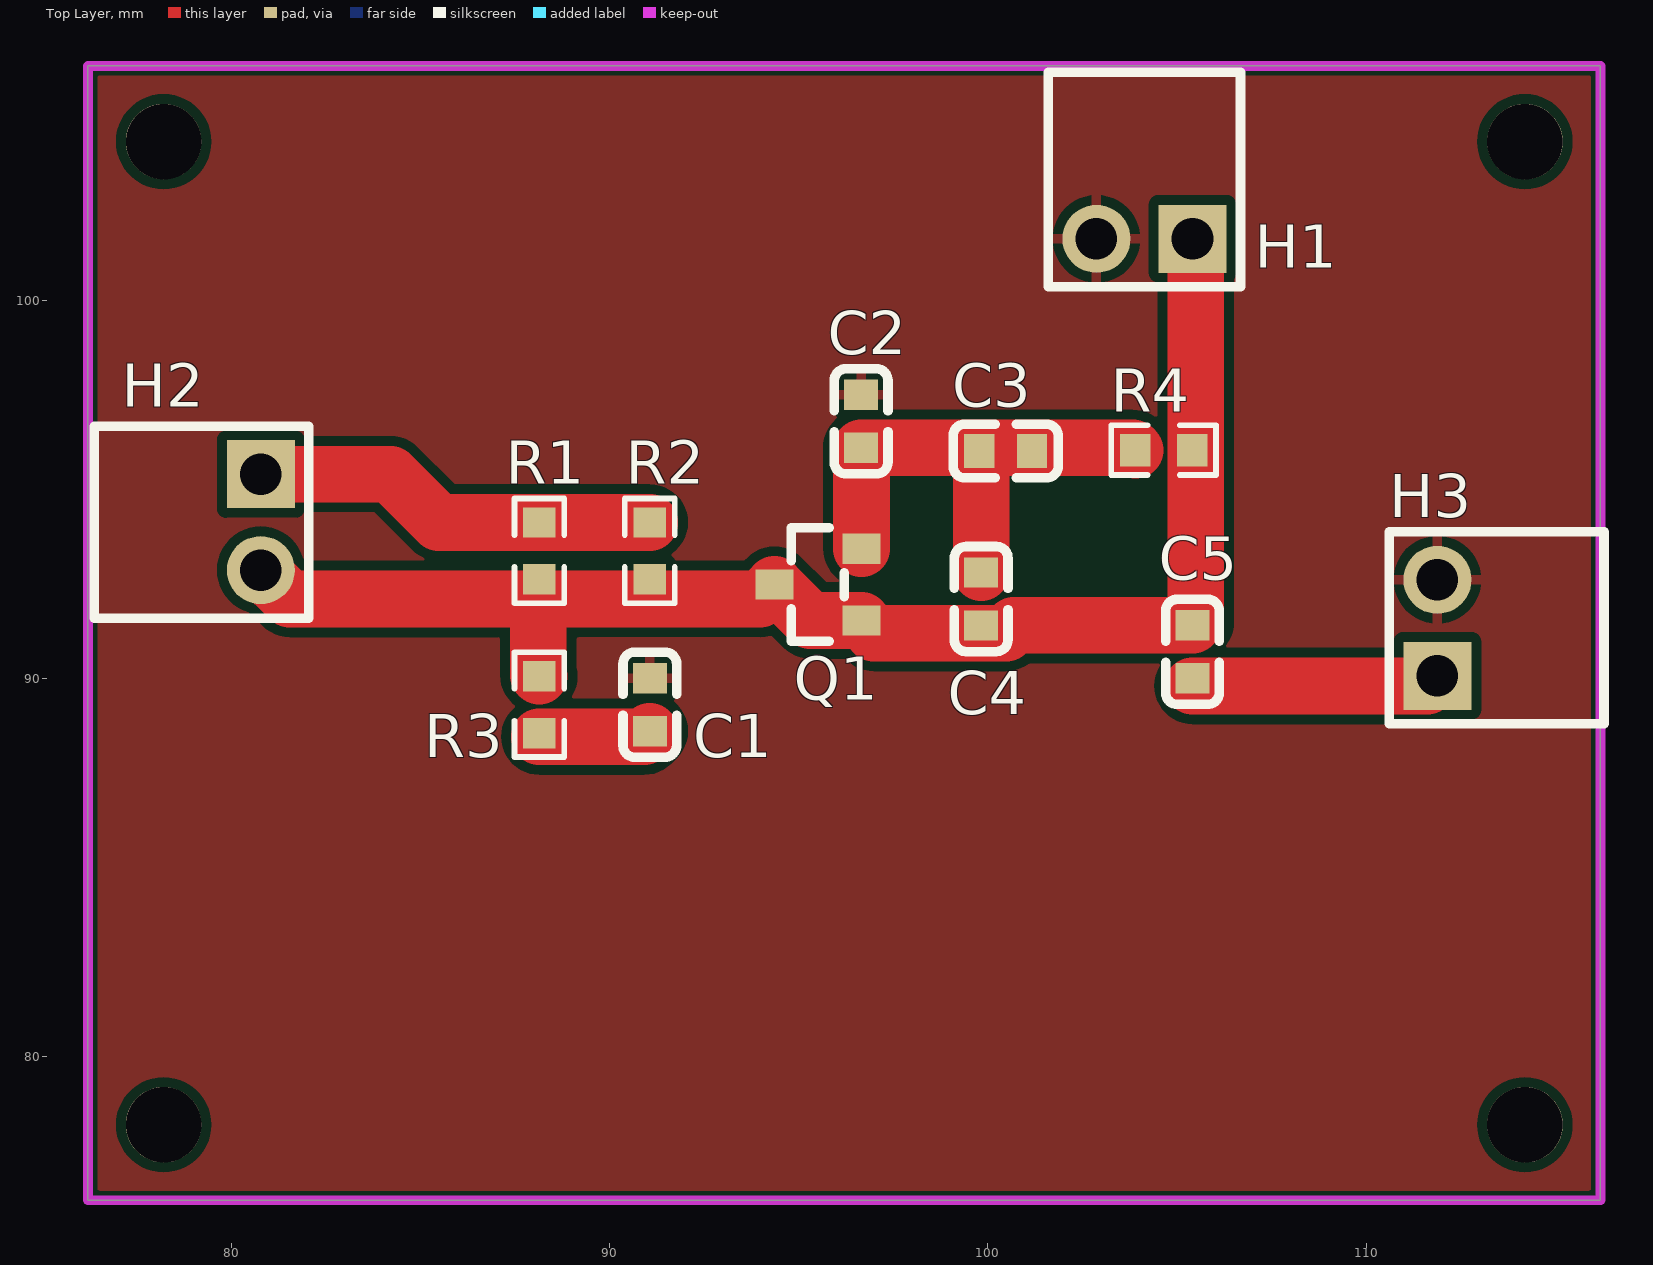
[diagram p0: Top Layer view]
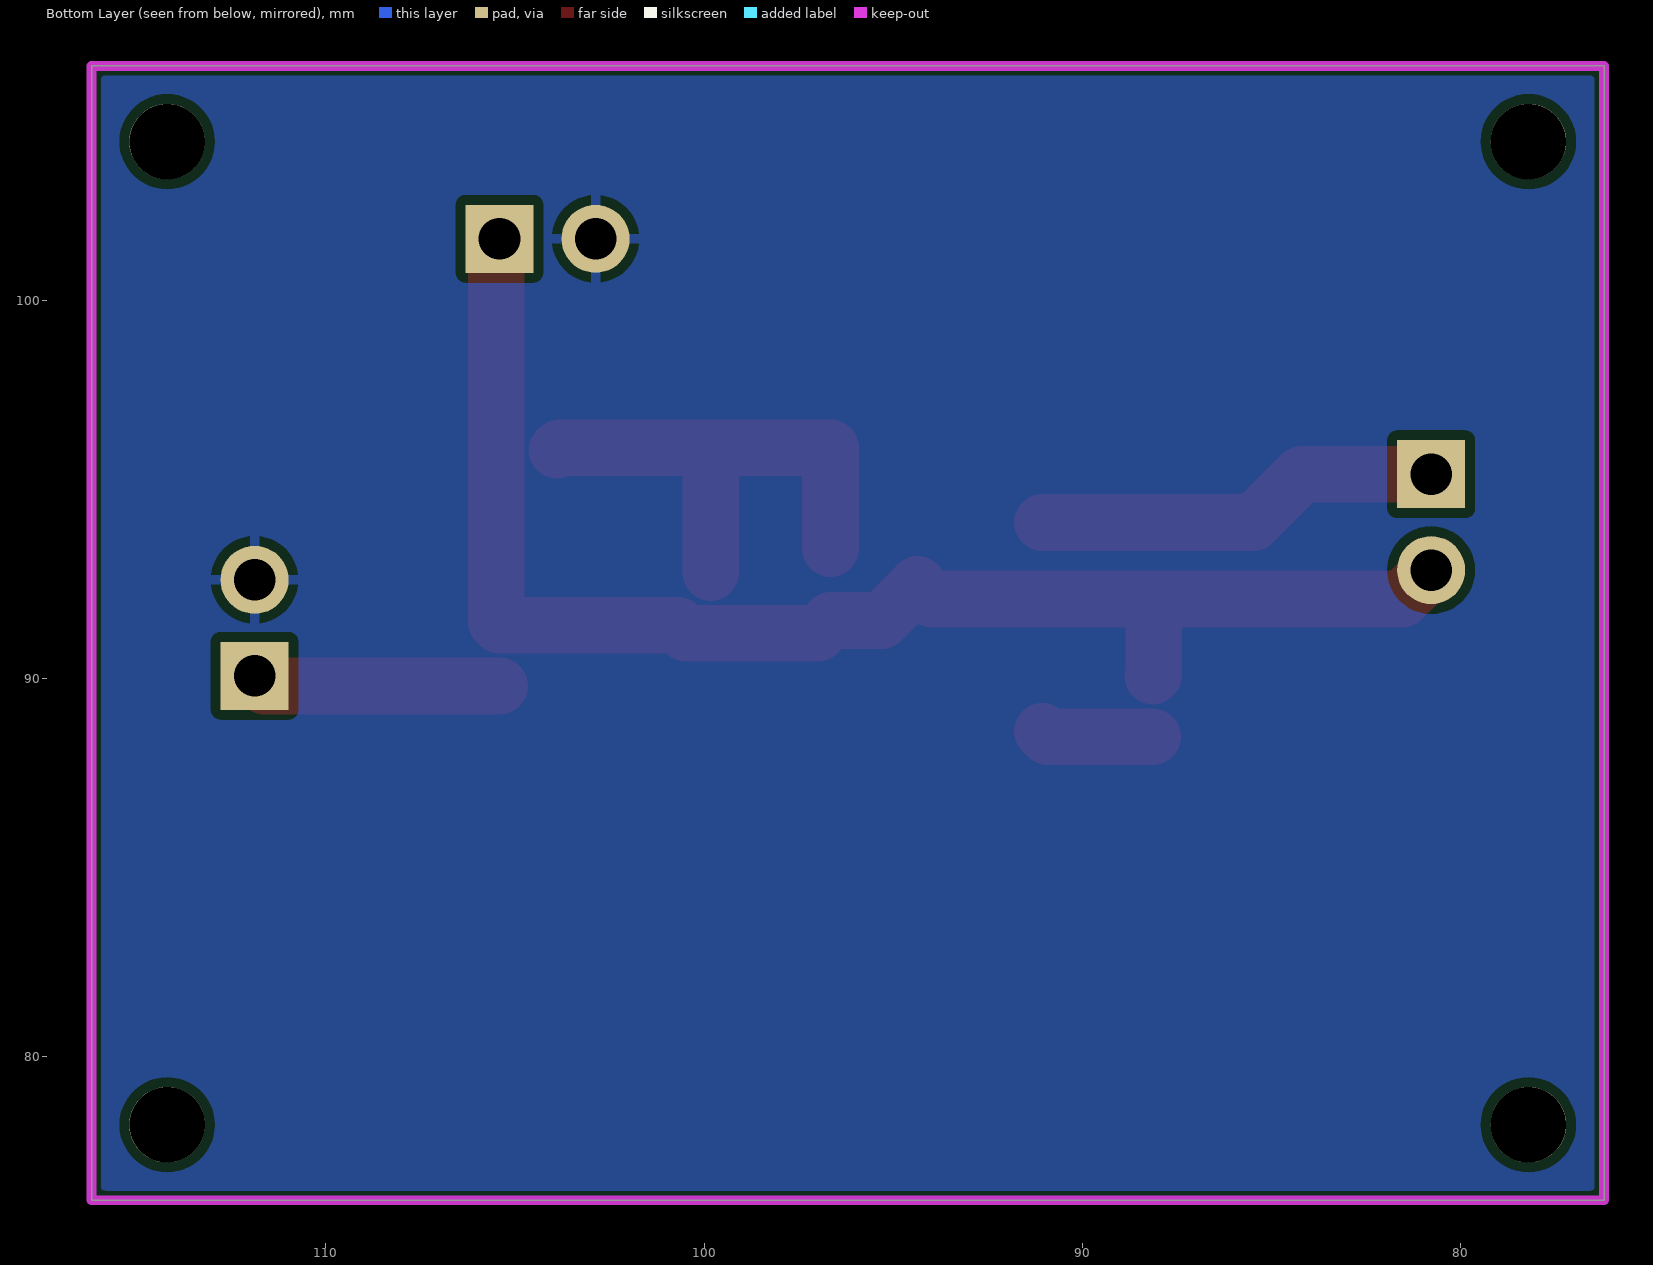
[diagram p1: Bottom Layer view, seen from below]
# Altium PCB MISC52148.pcbdoc
Units mm, origin at the board's own origin, x right, y up, seen from the top; angles counter-clockwise.
Board outline 40 x 30 mm, 2 copper layers (Top Layer, Bottom Layer), stack 1.58 mm thick; 13 components, 6 nets, 31 pads, 0 vias.

## Layer stack, top to bottom
Top Solder Mask Layer: solder mask 0.01, Dk 3.3
Top Layer: signal copper 0.035
Dielectric1: surface 1.51, FR4, Dk 4.5
Bottom Layer: signal copper 0.035
Bottom Solder Mask Layer: solder mask 0.01, Dk 3.3

## Board outline
76.2,106.2 76.2,76.2 116.2,76.2 116.2,106.2

## Design rules (kind name [scope] priority, off if disabled: settings)
BoardOutlineClearance copperThickness2oz_1 [All] p2 off: genericclearance=0.203 ignorepadtopadclearanceinfootprint=FALSE except(0: Arc-SplitContinuation Track-SplitContinuation SMDPad-SplitContinuation THPad-SplitContinuation Via-SplitContinuation Fill-SplitContinuation Region-SplitContinuation Poly-SplitContinuation Text-SplitContinuation Hole-SplitContinuation; 0.152: Arc-CutoutEdge SMDPad-CutoutEdge THPad-CutoutEdge Via-CutoutEdge Fill-CutoutEdge Region-CutoutEdge Text-CutoutEdge; 0.176: Hole-OutlineEdge Hole-CutoutEdge; 0.254: Poly-OutlineEdge Poly-CutoutEdge; 0.3: Arc-OutlineEdge Track-OutlineEdge SMDPad-OutlineEdge THPad-OutlineEdge Via-OutlineEdge Fill-OutlineEdge Region-OutlineEdge Text-OutlineEdge Track-CutoutEdge)
BoardOutlineClearance copperThickness1oz_1 [All] p4: genericclearance=0.102 ignorepadtopadclearanceinfootprint=FALSE except(0: Arc-SplitContinuation Track-SplitContinuation SMDPad-SplitContinuation THPad-SplitContinuation Via-SplitContinuation Fill-SplitContinuation Region-SplitContinuation Poly-SplitContinuation Text-SplitContinuation Hole-SplitContinuation; 0.152: SMDPad-CutoutEdge THPad-CutoutEdge Via-CutoutEdge Fill-CutoutEdge Region-CutoutEdge Text-CutoutEdge; 0.176: Hole-OutlineEdge Hole-CutoutEdge; 0.254: Poly-OutlineEdge Poly-CutoutEdge; 0.3: Arc-OutlineEdge Track-OutlineEdge SMDPad-OutlineEdge THPad-OutlineEdge Via-OutlineEdge Fill-OutlineEdge Region-OutlineEdge Text-OutlineEdge Arc-CutoutEdge Track-CutoutEdge)
Clearance copperThickness2oz [All] p1 off: gap=0.203 ignorepadtopadclearanceinfootprint=FALSE except(0.152: SMDPad-Track SMDPad-SMDPad THPad-Track SMDPad-THPad THPad-THPad Track-Via SMDPad-Via THPad-Via Via-Via Fill-Track Region-Track Fill-SMDPad Region-SMDPad Fill-THPad Region-THPad Fill-Via Region-Via Fill-Fill Fill-Region Region-Region Arc-Track Arc-SMDPad Arc-THPad Arc-Via Fill-Arc Region-Arc Arc-Arc Text-Track SMDPad-Text Text-THPad Text-Via Fill-Text Region-Text Arc-Text Text-Text; 0.176: Hole-Track Hole-SMDPad Hole-THPad Hole-Via Fill-Hole Region-Hole Hole-Arc Hole-Text; 0.254: Poly-Track Poly-SMDPad Poly-THPad Poly-Via Poly-Fill Poly-Region Poly-Poly Poly-Arc Poly-Text Poly-Hole)
Clearance copperThickness1oz [All] p3: gap=0.102 ignorepadtopadclearanceinfootprint=FALSE except(0.152: SMDPad-Track SMDPad-SMDPad THPad-Track SMDPad-THPad THPad-THPad Track-Via SMDPad-Via THPad-Via Via-Via Fill-Track Region-Track Fill-SMDPad Region-SMDPad Fill-THPad Region-THPad Fill-Via Region-Via Fill-Fill Fill-Region Region-Region Arc-Track Arc-SMDPad Arc-THPad Arc-Via Fill-Arc Region-Arc Arc-Arc Text-Track SMDPad-Text Text-THPad Text-Via Fill-Text Region-Text Arc-Text Text-Text; 0.176: Hole-Track Hole-SMDPad Hole-THPad Hole-Via Fill-Hole Region-Hole Hole-Arc Hole-Text; 0.254: Poly-Track Poly-SMDPad Poly-THPad Poly-Via Poly-Fill Poly-Region Poly-Poly Poly-Arc Poly-Text Poly-Hole)
Creepage creepage [All] p1: checkdistance=0 ignoreinternallayers=TRUE applytopolygonpour=TRUE
DiffPairsRouting differentialPair [All] p1: maxlimit=0.152 minlimit=0.152 mostfreqgap=0.152 toplayer_minwidth=0.127 toplayer_prefwidth=0.254 toplayer_maxwidth=2.54 toplayer_mingap=0.152 toplayer_prefgap=0.152 toplayer_maxgap=0.152 bottomlayer_minwidth=0.127 bottomlayer_prefwidth=0.254 bottomlayer_maxwidth=2.54 bottomlayer_mingap=0.152 bottomlayer_prefgap=0.152 bottomlayer_maxgap=0.152 maxuncoupledlength=0.254
HoleToHoleClearance otherClearance [All] p1: gap=0.3 allowstackedmicrovias=TRUE
Length netLength [All] p1: minlimit=0 maxlimit=0
MatchedLengths netLengthTolerance [All] p1: tolerance=25.4
PasteMaskExpansion pasteMaskExpansion [All] p1: expansion=0
PlaneConnect innerPlane [All] p1: planeconnectstyle=Relief reliefexpansion=0.508 reliefentries=4 reliefconductorwidth=0.254 reliefairgap=0.254
PolygonConnect copperRegion [(InNet('GND'))] p1: connectstyle=Relief reliefconductorwidth=0.254 reliefentries=4 polygonreliefangle="90 Angle" airgapwidth=0.254 via.connectstyle=Relief via.reliefconductorwidth=0.254 via.reliefentries=4 via.polygonreliefangle="90 Angle" via.airgapwidth=0.254
RoutingVias viaSize [All] p1: holewidth=0.305 width=0.61 viastyle="Through Hole" minholewidth=0.3 minwidth=0.5 maxholewidth=6.3 maxwidth=10
SolderMaskExpansion solderMaskExpansion [IsVia] p1: expansion=-25.4 istentingtop=TRUE
SolderMaskExpansion solderMaskExpansion [All] p2: expansion=0.051 istentingtop=FALSE
Width copperThickness2oz_2 [All] p1 off: maxlimit=2.54 minlimit=0.203 preferedwidth=0.254
Width copperThickness1oz_2 [All] p2: maxlimit=2.54 minlimit=0.127 preferedwidth=0.254

## Components (designator, comment, footprint, x,y, rotation, side; value= is the part's Value field where it differs from the comment)
C1 "20uF" C0603 91.059,89.309 r270 top
C2 "100nF" C0603 96.647,96.802 r270 top
C3 "100nF" C0603 100.469,96.017 r0 top
C4 "100nF" C0603 99.822,92.103 r270 top
C5 "20uF" C0603 105.41,90.706 r270 top
H1 "" HDR-TH_2P-P2.54-V-M-1 104.14,101.628 r180 top
H2 "" HDR-TH_2P-P2.54-V-M-1 80.772,94.135 r270 top
H3 "" HDR-TH_2P-P2.54-V-M-1 111.887,91.341 r90 top
Q1 "" S8050_SOT-23 95.504,92.484 r0 top
R1 "1K" R0603 88.138,93.373 r270 top
R2 "1K" R0603 91.059,93.373 r90 top
R3 "4.7K" R0603 88.138,89.309 r90 top
R4 "10K" R0603 104.648,96.04 r0 top

## Footprints (in the part's own frame and the unit in brackets; to place one, negate y for a bottom-side part, rotate by r counter-clockwise, add the part's x,y. Pads: shape width x height; smd on the part's side, far side on the other; paste and mask are expansions set on the pad)
C0603 [mm]
  rect 0.8x0.9 smd: 1(-0.7,0) 2(0.7,0)
  silkscreen extent -1.39,-0.71 1.39,0.71
HDR-TH_2P-P2.54-V-M-1 [mm]
  rect 1.8x1.8 hole 1.1: 1(-1.27,0)
  round 1.8 hole 1.1: 2(1.27,0)
  silkscreen extent -2.54,-4.41 2.54,1.27
R0603 [mm]
  rect 0.806x0.864 smd paste-100 mask+0.051: 1(-0.753,0) 2(0.753,0)
  silkscreen extent -1.39,-0.66 1.39,0.66
S8050_SOT-23 [mm]
  rect 1x0.8 smd paste+0 mask+0.051: 1(1.15,-0.95) 2(1.15,0.95) 3(-1.15,0)
  silkscreen extent -0.7,-1.5 0.7,1.5

## Free pads (board coordinates)
  round 2 hole 2: 1(78.2,78.2) 1(78.2,104.2) 1(114.2,78.2) 1(114.2,104.2)

## Nets (pads, with @x,y where several pads share a name; then routed paths per layer and width w, separated by ;. In a path a pad name is that pad's centre, name@x,y a point inside that pad or via, vN(x,y) a via of type N, cw(c..) or ccw(c..) an arc to the next point about the centre after c; other vN are vias at no path point)
$1N24: H2.1 R1.1 R2.2 | length 10.8
  Top Layer w1.5: H2.1 84.201,95.405 85.48,94.126 R1.1 R2.2
$1N26: C1.2 R3.1 | length 3
  Top Layer w1.5: R3.1@88.138,88.46 90.91,88.46 C1.2
$1N28: C2.2 C3.1 C3.2 C4.1 Q1.2 R4.1 | length 13.2
  Top Layer w1.5: Q1.2 96.654,96.095 C2.2 103.833,96.102 R4.1 ; C3.1 99.822,95.964 C4.1
$1N33: C5.2 H3.1 | length 6.6
  Top Layer w1.5: C5.2@105.41,89.804 111.62,89.804 H3.1
GND: C1.1 C2.1 H1.2 H3.2
VCC: C4.2 C5.1 H1.1 H2.2 Q1.1 Q1.3 R1.2 R2.1 R3.2 R4.2 | length 38.1
  Top Layer w1.5: H2.2 81.534,92.103 88.108,92.103 ; R3.2 88.108,90.092 88.108,92.103 ; H1.1 105.497,101.541 105.497,91.493 C5.1 100.691,91.406 100.486,91.201 96.987,91.201 Q1.1 95.304,91.534 Q1.3 93.973,92.103 88.108,92.103

## Polygon pours and split planes (outlines as drawn)
GND on Top Layer (solid, remove dead copper, pour order 0): 76.2,106.2 76.2,76.2 116.2,76.2 116.2,106.2
GND on Bottom Layer (solid, remove dead copper, pour order 2): 76.2,106.2 76.2,76.2 116.2,76.2 116.2,106.2

## Keep-outs
Board Outline Layer:
  the board outline again, w0.254